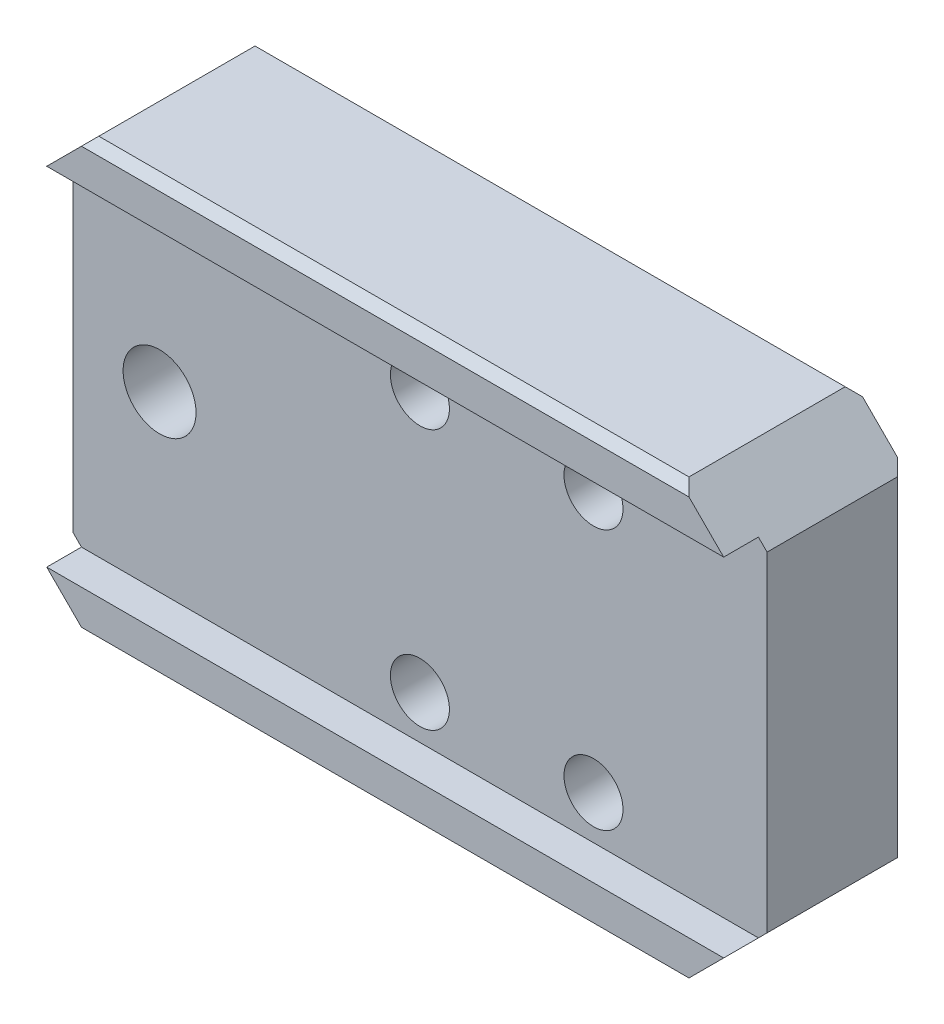
from build123d import *

# Parameters (mm, degrees)
SKETCH1_W                                          = 40
SKETCH1_H                                          = 25
BOSS_EXTRUDE1_DEPTH                                = 10
SKETCH2_W                                          = 40
SKETCH2_H                                          = 20
CUT_EXTRUDE1_DEPTH                                 = 2
M5_TAPPED_HOLE1_D                                  = 4.2
HOLE_SIZE_BASED_ON_SOCKET_HEAD_CAP_SCR_D           = 3.4
HOLE_SIZE_BASED_ON_SOCKET_HEAD_CAP_SCR_CBORE_D     = 6
HOLE_SIZE_BASED_ON_SOCKET_HEAD_CAP_SCR_CBORE_DEPTH = 3.4
CHAMFER1_SIZE                                      = 3
CHAMFER2_SIZE                                      = 0.5


with BuildPart() as part:
    # Sketch1 → Boss-Extrude1 (new body)
    with BuildSketch(Plane.XY):
        Rectangle(SKETCH1_W, SKETCH1_H)
    extrude(amount=BOSS_EXTRUDE1_DEPTH)

    # Sketch2 → Cut-Extrude1 (cut)
    with BuildSketch(Plane.XY.offset(10)):
        Rectangle(SKETCH2_W, SKETCH2_H)
    extrude(amount=-CUT_EXTRUDE1_DEPTH, mode=Mode.SUBTRACT)

    # M5 Tapped Hole1 (through all)
    with Locations(Plane.XY.offset(8)):
        with Locations((-15, 0)):
            Hole(M5_TAPPED_HOLE1_D / 2)

    # Hole Size (Based On) Socket Head Cap Screw Type1 (through all)
    with Locations(Plane(origin=(0, 0, 0), x_dir=(-1, 0, 0), z_dir=(0, 0, -1))):
        with Locations((-10, 7.5), (-10, -7.5), (0, 7.5), (0, -7.5)):
            CounterBoreHole(HOLE_SIZE_BASED_ON_SOCKET_HEAD_CAP_SCR_D / 2, HOLE_SIZE_BASED_ON_SOCKET_HEAD_CAP_SCR_CBORE_D / 2, HOLE_SIZE_BASED_ON_SOCKET_HEAD_CAP_SCR_CBORE_DEPTH)

    # Chamfer1
    chamfer1_edges = [part.edges().sort_by_distance(p)[0] for p in [
        (20, -12.5, 5),
        (20, 12.5, 5),
        (-20, -12.5, 5),
        (-20, 12.5, 5),
    ]]
    chamfer(chamfer1_edges, length=CHAMFER1_SIZE)

    # Chamfer2
    chamfer2_edges = [part.edges().sort_by_distance(p)[0] for p in [
        (20, 0, 0),
        (0, -12.5, 0),
        (-20, 0, 0),
        (0, 12.5, 0),
        (0, -12.5, 10),
        (0, 12.5, 10),
    ]]
    chamfer(chamfer2_edges, length=CHAMFER2_SIZE)


solid = part.part
